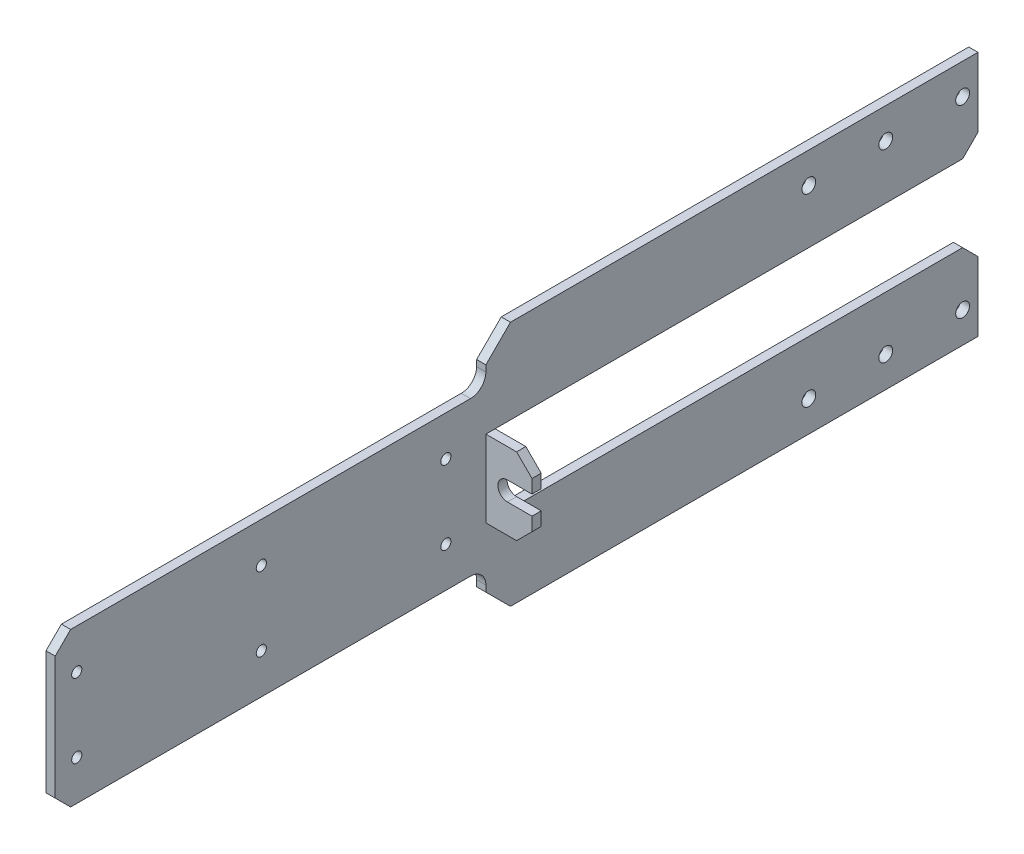
SolidWorks part; units mm, degrees
material "AISI 304"
ref_plane "Front Plane" through (0, 0, 0) normal (0, 0, 1) x (1, 0, 0)
ref_plane "Top Plane" through (0, 0, 0) normal (0, 1, 0) x (1, 0, 0)
ref_plane "Right Plane" through (0, 0, 0) normal (1, 0, 0) x (0, 0, -1)
sketch "Sketch1" plane through (0, 0, 0) normal (0, 1, 0) x (1, 0, 0)
  line L1 (0, 0) -> (18, 0)
  line L2 (0, 0) -> (0, 160)
  line L3 (0, 160) -> (3, 160)
  line L4 (18, 0) -> (18, 3)
  line L7 (18, 3) -> (3, 3)
  line L8 (3, 160) -> (3, 3)
  dimension "D1" = 3
  dimension "D2" = 3
  dimension "D3" = 18
  dimension "D4" = 160
extrude "Boss-Extrude1" add sketch "Sketch1" along normal blind 80
sketch "Sketch2" plane through (0, 0, 0) normal (0, 0, 1) x (1, 0, 0)
  line L0 (0, 40) -> (50000, 40) construction
  line L1 (0, 80) -> (0, 0) construction
  circle A0 centre (10, 40) radius 2.75
  point P4 (0, 40)
  dimension "D1" = 5.5
  dimension "D2" = 10
extrude "Cut-Extrude1" cut sketch "Sketch2" against normal blind 10
sketch "Sketch3" plane through (0, 0, 0) normal (-1, 0, 0) x (0, 0, 1)
  line L0 (-150, 40) -> (49850, 40) construction
  line L1 (-160, 80) -> (-160, 0) construction
  line L3 (-317, 27.5) -> (-3, 27.5)
  line L4 (-317, 27.5) -> (-317, 52.5)
  line L5 (-317, 52.5) -> (-3, 52.5)
  line L6 (-3, 27.5) -> (-3, 52.5)
  line L7 (-317, 27.5) -> (-3, 52.5) construction
  line L8 (-317, 52.5) -> (-3, 27.5) construction
  point P4 (-160, 40)
  point P5 (-160, 40)
  dimension "D1" = 25
  dimension "D2" = 157
extrude "Cut-Extrude2" cut sketch "Sketch3" against normal blind 10
sketch "Sketch4" plane through (0, 0, 0) normal (-1, 0, 0) x (0, 0, 1)
  line L0 (0, 40) -> (-50000, 40) construction
  line L1 (0, 80) -> (0, 0) construction
  line L3 (140, 15) -> (0, 15)
  line L4 (140, 15) -> (140, 65)
  line L5 (140, 65) -> (0, 65)
  line L6 (0, 15) -> (0, 65)
  line L7 (140, 15) -> (0, 65) construction
  line L8 (140, 65) -> (0, 15) construction
  point P4 (0, 40)
  point P5 (70, 40)
  dimension "D1" = 50
  dimension "D2" = 140
extrude "Boss-Extrude2" add sketch "Sketch4" against normal up to surface (3 mm away) up to face at (3, 13.75, -81.5)
sketch "Sketch5" plane through (18, 0, 0) normal (1, 0, 0) x (0, 0, -1)
  line L0 (10, 13.75) -> (50010, 13.75) construction
  line L1 (10, 27.5) -> (-14.7123, 27.5)
  line L2 (-135, 40) -> (49865, 40) construction
  line L3 (10, 0) -> (-14.7123, 0)
  line L4 (-140, 65) -> (-140, 15) construction
  line L5 (3, 27.5) -> (3, 0) construction
  line L6 (-14.7123, 0) -> (-14.7123, 27.5)
  line L7 (10, 66.25) -> (50010, 66.25) construction
  line L8 (10, 0) -> (10, 27.5)
  line L9 (10, 80) -> (10, 52.5)
  line L11 (-14.7123, 80) -> (-14.7123, 52.5)
  line L12 (10, 80) -> (-14.7123, 80)
  line L13 (10, 52.5) -> (-14.7123, 52.5)
  point P9 (3, 13.75)
  point P14 (-140, 40)
extrude "Cut-Extrude3" cut sketch "Sketch5" against normal up to surface (15 mm away) up to face at (3, 13.75, -81.5)
chamfer "Chamfer1" distance 5 angle 45 2 edges at (18, 52.5, -1.5) (18, 27.5, -1.5)
chamfer "Chamfer2" distance 8 angle 45 2 edges at (1.5, 0, 0) (1.5, 80, 0)
sketch "Sketch8" plane through (0, 0, -3) normal (0, 0, -1) x (-1, 0, 0)
  line L0 (-17, 40) -> (49983, 40) construction
  line L1 (-18, 47.5) -> (-18, 32.5) construction
  line L2 (-26, 40) -> (-10, 40) construction
  line L3 (-26, 43.1) -> (-10, 43.1)
  line L4 (-26, 36.9) -> (-10, 36.9)
  arc A0 (-26, 43.1) -> (-26, 36.9) centre (-26, 40) ccw
  arc A1 (-10, 36.9) -> (-10, 43.1) centre (-10, 40) ccw
  point P4 (-18, 40)
  point P7 (-18, 40)
  dimension "D2" = 8
  dimension "D1" = 6.2
extrude "Cut-Extrude4" cut sketch "Sketch8" against normal blind 112
sketch "Sketch9" plane through (0, 0, 0) normal (-1, 0, 0) x (0, 0, 1)
  line L0 (180, 40) -> (-49820, 40) construction
  line L1 (140, 15) -> (140, 65) construction
  circle A0 centre (133, 52) radius 1
  circle A1 centre (133, 28) radius 1
  point P4 (140, 40)
  dimension "D3" = 2
  dimension "D1" = 24
  dimension "D2" = 7
extrude "Cut-Extrude5" cut sketch "Sketch9" against normal blind 10
hole_wizard "M4 Tapped Hole1" positions "3DSketch1" profile "Sketch10" tap size "M4" standard "Gb"
sketch3d "3DSketch1"
  line L0 (3, 52, 133) -> (0, 52, 133) construction
  line L1 (3, 28, 133) -> (0, 28, 133) construction
  point P0 (0, 52, 133)
  point P4 (0, 28, 133)
sketch "Sketch10" plane through (0, 52, 133) normal (0, 1, 0) x (0, 0, 1)
  line L0 (0, 0) -> (0, 11.0914)
  line L1 (0, 11.0914) -> (1.65, 10.1)
  line L2 (1.65, 10.1) -> (1.65, 0)
  line L5 (1.65, 0) -> (0, 0)
  line L10 (0, 11.0914) -> (-1.65, 10.1) construction
  line L11 (0, -6.35) -> (0, 107.95) construction
  dimension "螺纹孔钻头直径" = 3.3
  dimension "螺纹孔钻头深度" = 10.1
  dimension "导头角度" = 118
cosmetic thread "Cosmetic thread 1" parameters "D1"=3, "D2"=4
cosmetic thread "Cosmetic thread 2" parameters "D1"=3, "D2"=4
pattern_linear "LPattern1" count 3 spacing 60 along (0, 0, -1) of "M4 Tapped Hole1"
sketch "Sketch11" plane through (0, 0, 0) normal (-1, 0, 0) x (0, 0, 1)
  line L0 (180, 40) -> (-49820, 40) construction
  line L1 (140, 15) -> (140, 65) construction
  line L2 (-160, 80) -> (-160, 52.5) construction
  circle A0 centre (-155, 70) radius 2.25
  circle A1 centre (-155, 10) radius 2.25
  point P4 (140, 40)
  dimension "D1" = 4.5
  dimension "D2" = 5
  dimension "D3" = 60
extrude "Cut-Extrude6" cut sketch "Sketch11" against normal blind 10
pattern_linear "LPattern2" count 3 spacing 25 along (0, 0, 1) of "Cut-Extrude6"
chamfer "Chamfer3" distance 5 angle 45 2 edges at (1.5, 27.5, -160) (1.5, 52.5, -160)
chamfer "Chamfer4" distance 5 angle 45 2 edges at (1.5, 15, 140) (1.5, 65, 140)
fillet "Fillet1" radius 5 2 edges
